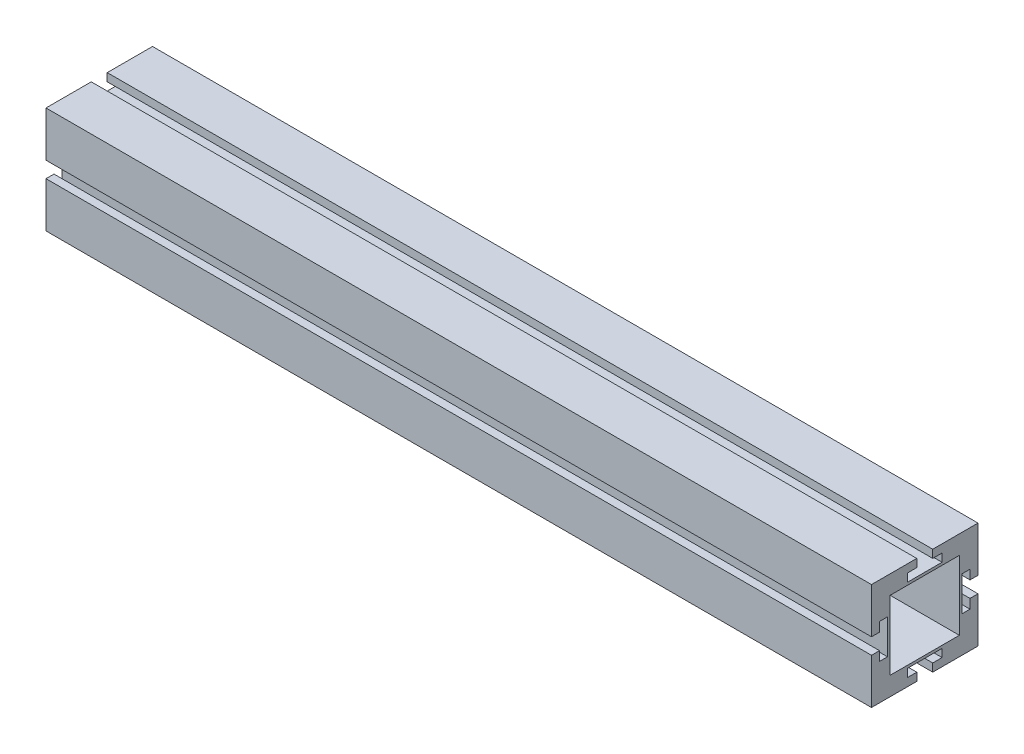
SolidWorks part; units mm, degrees
ref_plane "Front Plane" through (0, 0, 0) normal (0, 0, 1) x (1, 0, 0)
ref_plane "Top Plane" through (0, 0, 0) normal (0, 1, 0) x (1, 0, 0)
ref_plane "Right Plane" through (0, 0, 0) normal (1, 0, 0) x (0, 0, -1)
sketch "Sketch1" plane through (0, 0, 0) normal (1, 0, 0) x (0, 0, -1)
  line L0 (0, 0) -> (0, 33.8923) construction
  line L1 (-20, -20) -> (-3, -20)
  line L2 (-20, -20) -> (-20, -3)
  line L3 (-20, 20) -> (-3, 20)
  line L4 (20, -20) -> (20, -3)
  line L5 (-20, -20) -> (20, 20) construction
  line L6 (-20, 20) -> (20, -20) construction
  line L7 (-13, -13) -> (13, -13)
  line L8 (-13, -13) -> (-13, 13)
  line L9 (-13, 13) -> (13, 13)
  line L10 (13, -13) -> (13, 13)
  line L11 (-13, -13) -> (13, 13) construction
  line L12 (-13, 13) -> (13, -13) construction
  line L13 (0, 0) -> (25.505, 0) construction
  line L14 (17, 3) -> (17, 6.5)
  line L15 (-6.5, 17) -> (-3, 17)
  line L16 (6.5, 17) -> (6.5, 14)
  line L17 (3, 17) -> (6.5, 17)
  line L18 (-6.5, 14) -> (6.5, 14)
  line L19 (17, -6.5) -> (17, -3)
  line L20 (3, 20) -> (20, 20)
  line L21 (14, -6.5) -> (17, -6.5)
  line L22 (-3, 20) -> (-3, 17)
  line L23 (17, 3) -> (20, 3)
  line L24 (3, 20) -> (3, 17)
  line L25 (17, -3) -> (20, -3)
  line L26 (-20, 20) -> (20, 20) construction
  line L27 (14, -6.5) -> (14, 6.5)
  line L28 (-17, -17) -> (17, -17) construction
  line L29 (20, 3) -> (20, 20)
  line L30 (-6.5, 17) -> (-6.5, 14)
  line L31 (14, 6.5) -> (17, 6.5)
  line L32 (14, -14) -> (14, 14) construction
  line L33 (-14, 14) -> (14, 14) construction
  line L34 (-17, 17) -> (17, 17) construction
  line L35 (3, -20) -> (3, -17)
  line L36 (-17, -17) -> (-17, 17) construction
  line L37 (-14, -14) -> (-14, 14) construction
  line L38 (-14, -14) -> (14, -14) construction
  line L39 (17, -17) -> (17, 17) construction
  line L40 (20, -20) -> (20, 20) construction
  line L41 (3, -17) -> (6.5, -17)
  line L42 (6.5, -17) -> (6.5, -14)
  line L43 (-6.5, -14) -> (6.5, -14)
  line L44 (-6.5, -17) -> (-6.5, -14)
  line L45 (-6.5, -17) -> (-3, -17)
  line L46 (-3, -20) -> (-3, -17)
  line L47 (-14, -6.5) -> (-14, 6.5)
  line L48 (-14, -6.5) -> (-17, -6.5)
  line L49 (-17, -6.5) -> (-17, -3)
  line L50 (-17, -3) -> (-20, -3)
  line L51 (-17, 3) -> (-20, 3)
  line L52 (-17, 3) -> (-17, 6.5)
  line L53 (-14, 6.5) -> (-17, 6.5)
  line L54 (-20, 3) -> (-20, 20)
  line L55 (3, -20) -> (20, -20)
  line L56 (-20, -20) -> (-20, 20) construction
  line L58 (-20, -20) -> (20, -20) construction
  point P0 (0, 0)
  point P6 (0, 0)
  dimension "D1" = 40
  dimension "D2" = 40
  dimension "D3" = 26
  dimension "D4" = 26
  dimension "D7" = 3
  dimension "D8" = 3
  dimension "D9" = 6
  dimension "D10" = 13
  dimension "D11" = 3
  dimension "D12" = 6
  dimension "D13" = 13
  dimension "D5" = 3
  dimension "D6" = 3
extrude "Boss-Extrude1" add sketch "Sketch1" along normal blind 310
